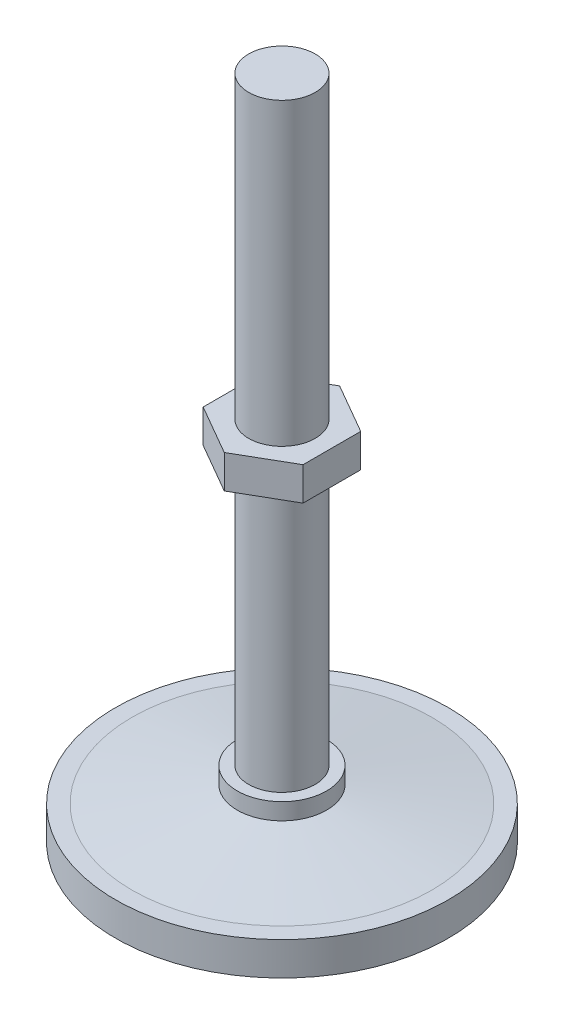
from build123d import *

# Parameters (mm, degrees)
EXTRUDE1_DEPTH = 10


with BuildPart() as part:
    # Sketch1 → Revolve1 (revolve)
    with BuildSketch(Plane.XY, mode=Mode.PRIVATE) as revolve1_sk:
        Polygon((0, 0), (50, 0), (50, 10), (45, 10), (13.404628949, 15), (13.404628949, 20), (10, 20), (10, 200), (0, 200), align=None)
    revolve(revolve1_sk.sketch.rotate(Axis((0, 0, 0), (0, 1, 0)), 90), axis=Axis((0, 0, 0), (0, 1, 0)))

    # Sketch2 → Extrude1 (add)
    with BuildSketch(Plane.XZ.offset(-110)):
        Polygon((0, 17.320508076), (-15, 8.660254038), (-15, -8.660254038), (0, -17.320508076), (15, -8.660254038), (15, 8.660254038), align=None)
    extrude(amount=EXTRUDE1_DEPTH)


solid = part.part
